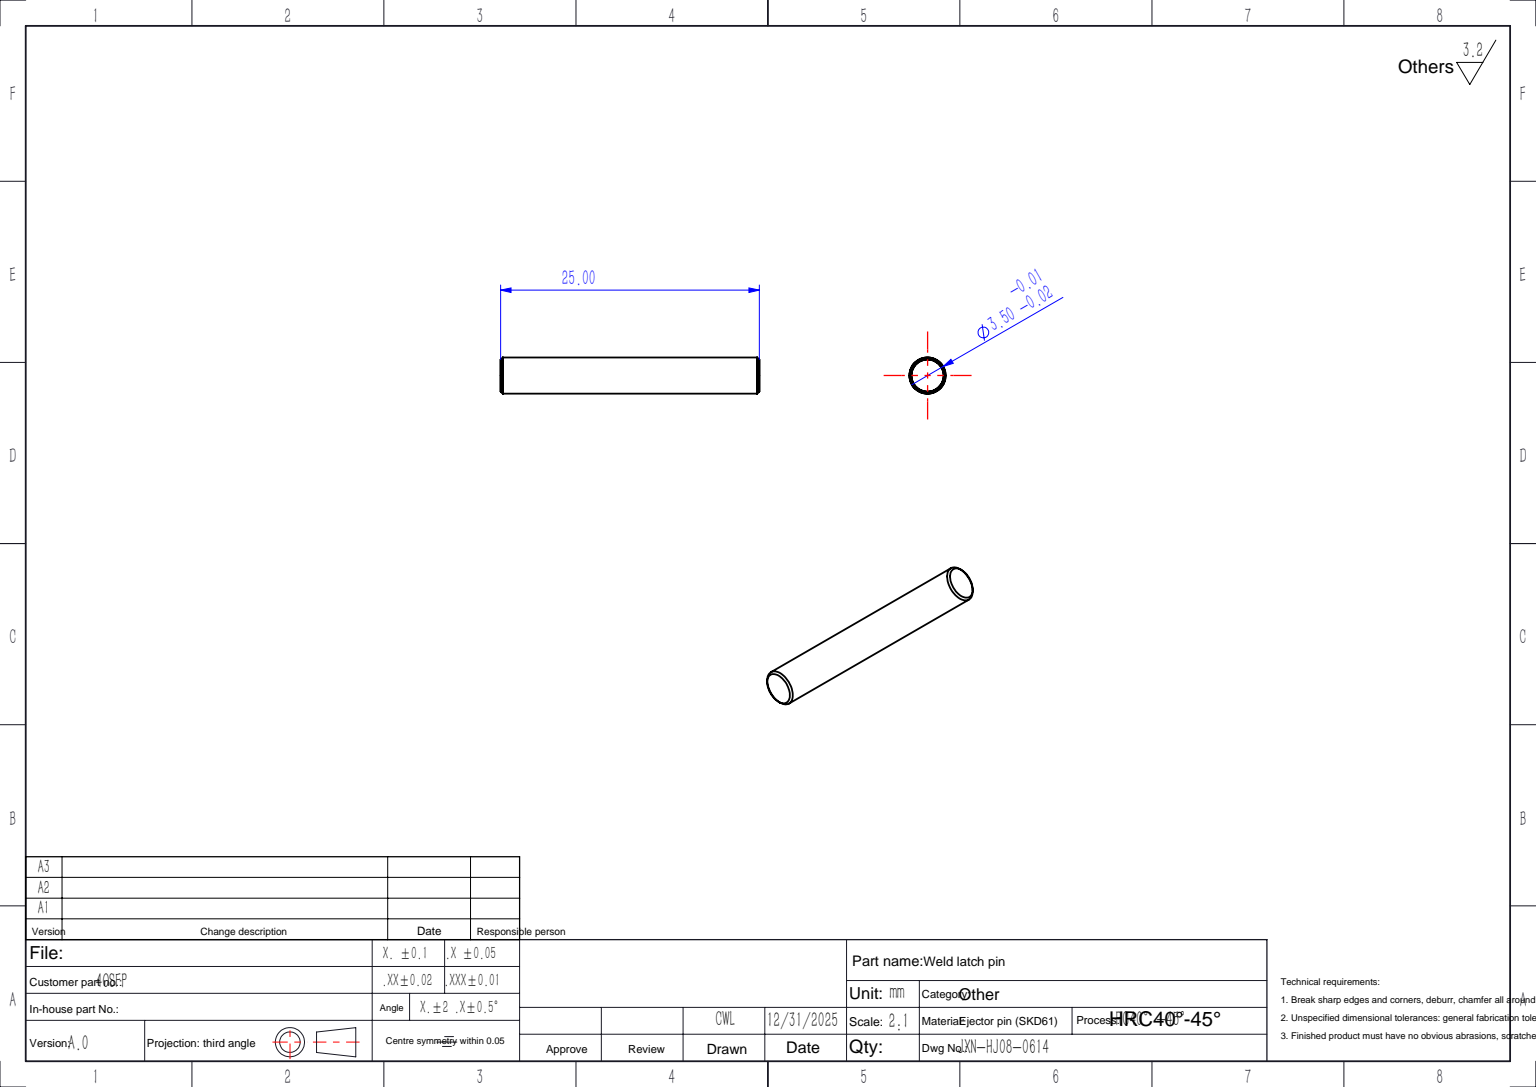
SolidWorks part; units mm, degrees
ref_plane "前视基准面" through (0, 0, 0) normal (0, 0, 1) x (1, 0, 0)
ref_plane "上视基准面" through (0, 0, 0) normal (0, 1, 0) x (1, 0, 0)
ref_plane "右视基准面" through (0, 0, 0) normal (1, 0, 0) x (0, 0, -1)
sketch "草图1" plane through (0, 0, 0) normal (0, 1, 0) x (1, 0, 0)
  circle A0 centre (0, 0) radius 1.75
  dimension "D1" = 3.5
extrude "凸台-拉伸1" add sketch "草图1" along normal blind 25
chamfer "倒角1" distance 0.2 angle 45 2 edges at (0, 25, 1.75) (0, 0, 1.75)
equation "\"code1\"= \"图名分离代码\""
equation "\"code2\"= \"图号分离代码\""
